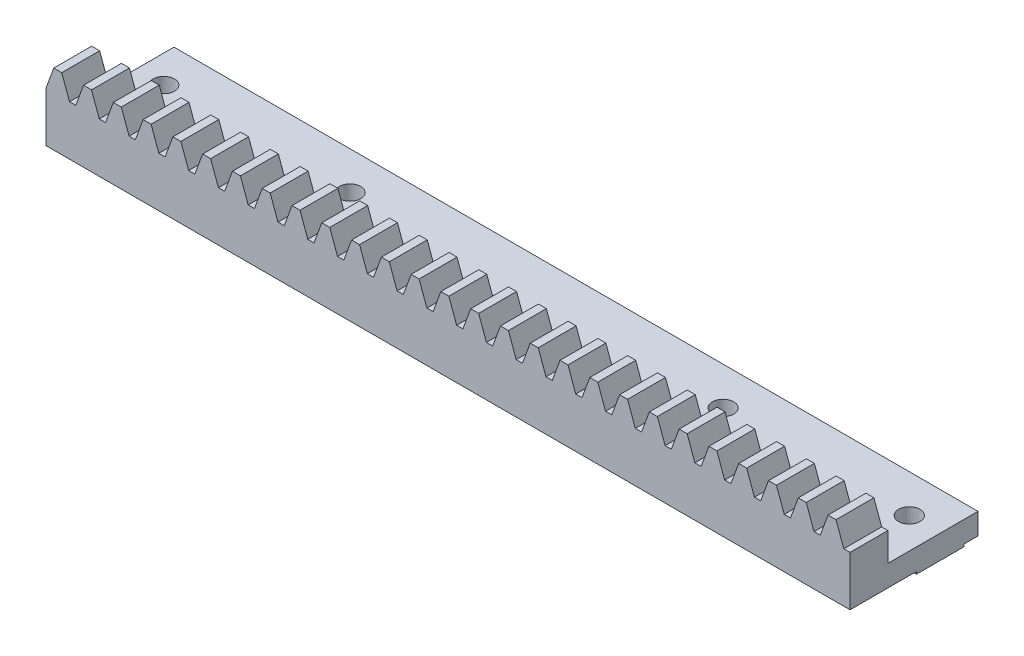
from build123d import *

# Parameters (mm, degrees)
SKETCH1_W              = 169.646003294
SKETCH1_H              = 11
EXTRUDE1_DEPTH         = 27
EXTRUDE2_DEPTH         = 8
LPATTERN1_COUNT        = 27
LPATTERN1_PITCH        = 6.283185307
SKETCH_1_W             = 169.646003294
SKETCH_1_H             = 19
CUT_EXTRUDE_1_DEPTH    = 6
SKETCH_3_R             = 2.25
CUT_EXTRUDE_2_DEPTH    = 10.5
PATTERN_LINEAR_2_COUNT = 2
PATTERN_LINEAR_2_PITCH = 118
SKETCH_5_W             = 169.646003294
SKETCH_5_H             = 14
SKETCH_5_H_2           = 3
CUT_EXTRUDE_3_DEPTH    = 0.5


with BuildPart() as part:
    # Sketch1 → Extrude1 (new body)
    with BuildSketch(Plane.XY):
        with Locations((84.823001647, -5.5)):
            Rectangle(SKETCH1_W, SKETCH1_H)
    extrude(amount=EXTRUDE1_DEPTH)

    # Sketch2 → Extrude2 (add)
    with BuildSketch(Plane.XY.offset(27)):
        Polygon((0, 0), (1.637866054, 4.5), (3.323577771, 4.5), (4.961443825, 0), align=None)
    extrude2 = extrude(amount=-EXTRUDE2_DEPTH)

    # LPattern1: Extrude2 ×27
    with Locations(*[(i * LPATTERN1_PITCH, 0, 0) for i in range(1, LPATTERN1_COUNT)]):
        add(extrude2)

    # 草图1 → 切除-拉伸1 (cut)
    with BuildSketch(Plane(origin=(0, 0, 0), x_dir=(1, 0, 0), z_dir=(0, 1, 0))):
        with Locations((84.823001647, -9.5)):
            Rectangle(SKETCH_1_W, SKETCH_1_H)
    extrude(amount=-CUT_EXTRUDE_1_DEPTH, mode=Mode.SUBTRACT)

    # 草图3 → 切除-拉伸2 (cut)
    with BuildSketch(Plane(origin=(0, -6, 0), x_dir=(1, 0, 0), z_dir=(0, 1, 0))):
        with Locations(Location((5.857142857, -8, 0), (0, 0, 270))):
            Circle(SKETCH_3_R)
        with Locations(Location((45.142857143, -8, 0), (0, 0, 270))):
            Circle(SKETCH_3_R)
    cut_extrude_2 = extrude(amount=-CUT_EXTRUDE_2_DEPTH, mode=Mode.SUBTRACT)

    # 阵列(线性)2: 切除-拉伸2 ×2
    with Locations(*[(i * PATTERN_LINEAR_2_PITCH, 0, 0) for i in range(1, PATTERN_LINEAR_2_COUNT)]):
        add(cut_extrude_2, mode=Mode.SUBTRACT)

    # 草图5 → 切除-拉伸3 (cut)
    with BuildSketch(Plane.XZ.offset(11)):
        with Locations((84.823001647, 20)):
            Rectangle(SKETCH_5_W, SKETCH_5_H)
        with Locations((84.823001647, 1.5)):
            Rectangle(SKETCH_5_W, SKETCH_5_H_2)
    extrude(amount=-CUT_EXTRUDE_3_DEPTH, mode=Mode.SUBTRACT)


solid = part.part
